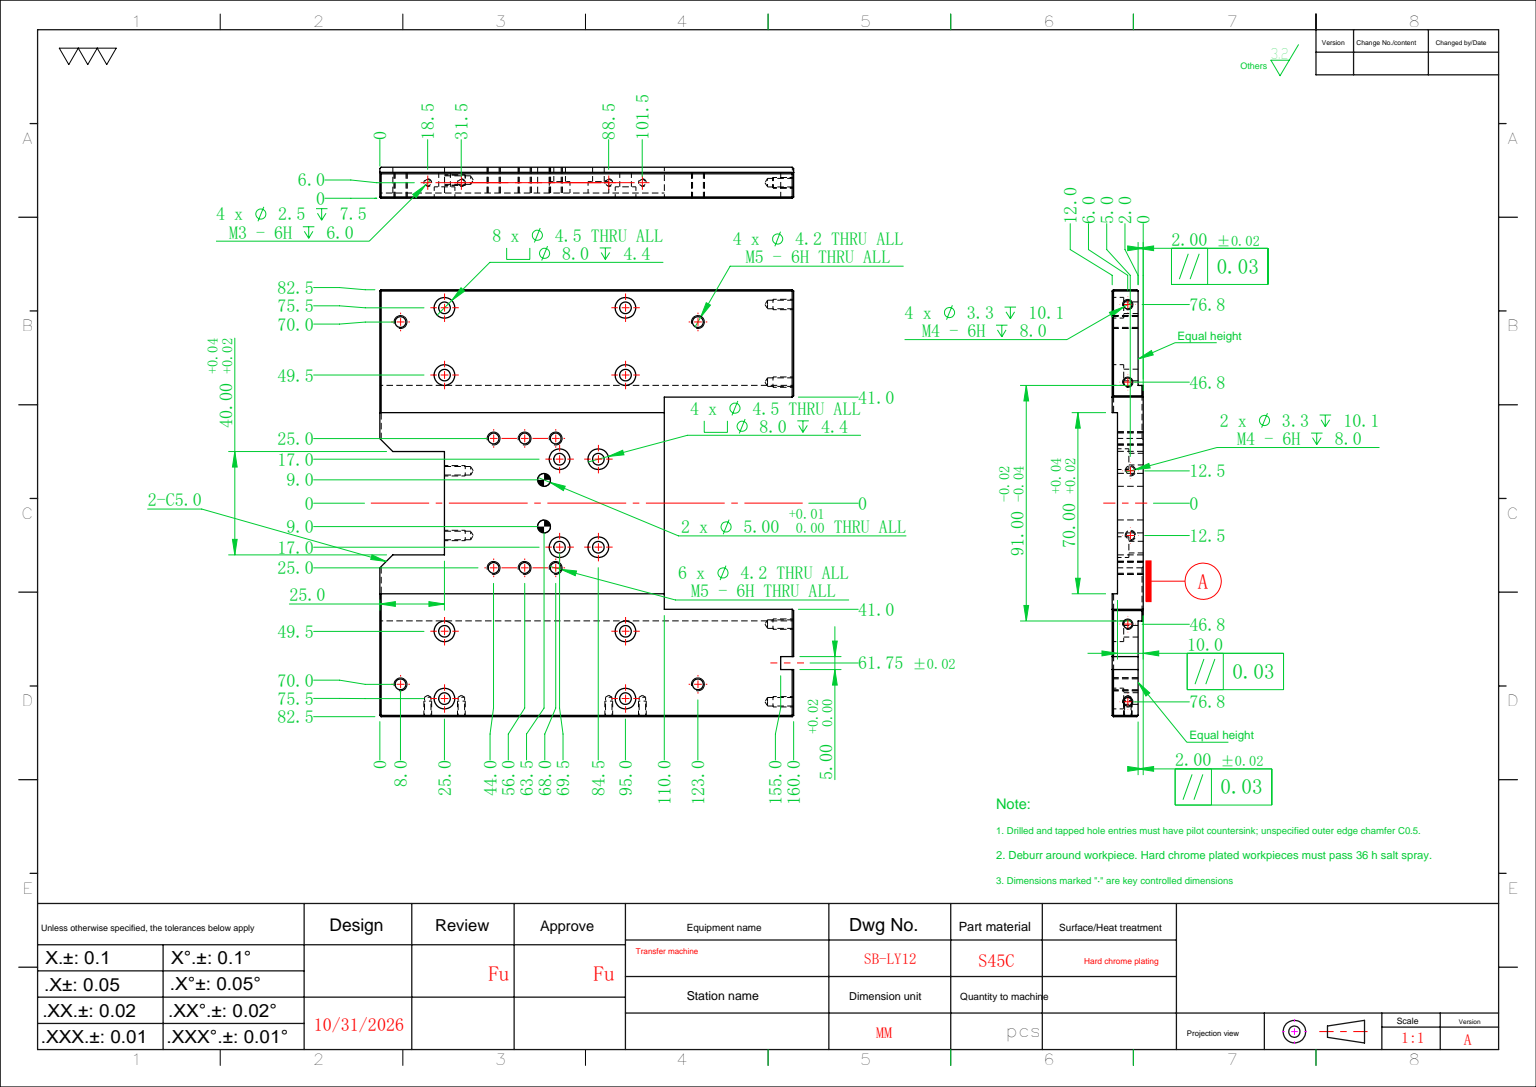
from build123d import *

# Parameters (mm, degrees)
SKETCH_1_W                   = 160
SKETCH_1_H                   = 165
EXTRUDE_1_DEPTH              = 12
SKETCH_2_W                   = 50
SKETCH_2_H                   = 82
CUT_EXTRUDE_1_DEPTH          = 116.543281934
SKETCH_3_W                   = 2
SKETCH_3_H                   = 34
CUT_EXTRUDE_2_DEPTH          = 181.416878368
HOLE_WIZARD_M4_2_D           = 4.5
HOLE_WIZARD_M4_2_CBORE_D     = 8
HOLE_WIZARD_M4_2_CBORE_DEPTH = 4.4
SKETCH_6_W                   = 110
SKETCH_6_H                   = 70
CUT_EXTRUDE_3_DEPTH          = 2
HOLE_WIZARD_M4_1_D           = 4.5
HOLE_WIZARD_M4_1_CBORE_D     = 8
HOLE_WIZARD_M4_1_CBORE_DEPTH = 4.4
MM_2_D                       = 5
HOLE_WIZARD_M5_1_D           = 4.2
HOLE_WIZARD_M4_1_2_D         = 3.3
HOLE_WIZARD_M4_1_2_DEPTH     = 10.1
HOLE_WIZARD_M4_1_2_TIP       = 0.991420021
SKETCH_17_W                  = 10
SKETCH_17_H                  = 5
CUT_EXTRUDE_4_DEPTH          = 5
HOLE_WIZARD_M5_2_D           = 4.2
PATTERN_LINEAR_1_COUNT       = 3
PATTERN_LINEAR_1_PITCH       = 12
SKETCH_20_W                  = 25
SKETCH_20_H                  = 40
CUT_EXTRUDE_5_DEPTH          = 116.543281934
CHAMFER_1_SIZE               = 5
HOLE_WIZARD_M4_2_2_D         = 3.3
HOLE_WIZARD_M4_2_2_DEPTH     = 10.1
HOLE_WIZARD_M4_2_2_TIP       = 0.991420021
HOLE_WIZARD_M3_1_AT_2_COUNT  = 2
HOLE_WIZARD_M3_1_AT_2_PITCH  = 13
PATTERN_LINEAR_2_COUNT       = 2
PATTERN_LINEAR_2_PITCH       = 70
SKETCH_25_W                  = 2
SKETCH_25_H                  = 3
CUT_EXTRUDE_6_DEPTH          = 181.416878368
CHAMFER_2_SIZE               = 0.5


with BuildPart() as part:
    # 草图1 → 凸台-拉伸1 (new body)
    with BuildSketch(Plane.XY):
        Rectangle(SKETCH_1_W, SKETCH_1_H)
    extrude(amount=EXTRUDE_1_DEPTH)

    # 草图2 → 切除-拉伸1 (cut, through all)
    with BuildSketch(Plane(origin=(0, 0, 0), x_dir=(-1, 0, 0), z_dir=(0, 0, -1))):
        with Locations((-55, 0)):
            Rectangle(SKETCH_2_W, SKETCH_2_H)
    extrude(amount=-CUT_EXTRUDE_1_DEPTH, mode=Mode.SUBTRACT)

    # 草图3 → 切除-拉伸2 (cut, through all)
    with BuildSketch(Plane.ZY.offset(80)):
        with Locations((11, 62.5)):
            Rectangle(SKETCH_3_W, SKETCH_3_H)
        with Locations((11, -62.5)):
            Rectangle(SKETCH_3_W, SKETCH_3_H)
    extrude(amount=-CUT_EXTRUDE_2_DEPTH, mode=Mode.SUBTRACT)

    # Hole Wizard M4 _2 (through all)
    with Locations(Plane(origin=(0, 0, 0), x_dir=(-1, 0, 0), z_dir=(0, 0, -1))):
        with Locations((-15, 49.5), (-15, 75.5), (-15, -75.5), (-15, -49.5), (55, -75.5), (55, -49.5), (55, 49.5), (55, 75.5)):
            CounterBoreHole(HOLE_WIZARD_M4_2_D / 2, HOLE_WIZARD_M4_2_CBORE_D / 2, HOLE_WIZARD_M4_2_CBORE_DEPTH)

    # 草图6 → 切除-拉伸3 (cut)
    with BuildSketch(Plane(origin=(0, 0, 0), x_dir=(-1, 0, 0), z_dir=(0, 0, -1))):
        with Locations((25, 0)):
            Rectangle(SKETCH_6_W, SKETCH_6_H)
    extrude(amount=-CUT_EXTRUDE_3_DEPTH, mode=Mode.SUBTRACT)

    # Hole Wizard M4 _1 (through all)
    with Locations(Plane(origin=(0, 0, 2), x_dir=(-1, 0, 0), z_dir=(0, 0, -1))):
        with Locations((-4.5, -17), (-4.5, 17), (10.5, -17), (10.5, 17)):
            CounterBoreHole(HOLE_WIZARD_M4_1_D / 2, HOLE_WIZARD_M4_1_CBORE_D / 2, HOLE_WIZARD_M4_1_CBORE_DEPTH)

    # 大小mm 暗销孔2 (through all)
    with Locations(Plane(origin=(0, 0, 2), x_dir=(-1, 0, 0), z_dir=(0, 0, -1))):
        with Locations((16.5, -9), (16.5, 9)):
            Hole(MM_2_D / 2)

    # M5 螺纹孔1 (through all)
    with Locations(Plane(origin=(0, 0, 0), x_dir=(-1, 0, 0), z_dir=(0, 0, -1))):
        with Locations((72, 70), (-43, 70), (-43, -70), (72, -70)):
            Hole(HOLE_WIZARD_M5_1_D / 2)

    # Hole Wizard M4 _1 2
    with Locations(Plane(origin=(80, 0, 0), x_dir=(0, 0, -1), z_dir=(1, 0, 0))):
        with Locations((-6, 76.75), (-6, 46.75), (-6, -46.75), (-6, -76.75)):
            Hole(HOLE_WIZARD_M4_1_2_D / 2, depth=HOLE_WIZARD_M4_1_2_DEPTH)
            with Locations((0, 0, -(HOLE_WIZARD_M4_1_2_DEPTH + HOLE_WIZARD_M4_1_2_TIP / 2))):  # 118° drill point
                Cone(0, HOLE_WIZARD_M4_1_2_D / 2, HOLE_WIZARD_M4_1_2_TIP, mode=Mode.SUBTRACT)

    # 草图17 → 切除-拉伸4 (cut)
    with BuildSketch(Plane(origin=(80, 0, 0), x_dir=(0, 0, -1), z_dir=(1, 0, 0))):
        with Locations((-5, 61.75)):
            Rectangle(SKETCH_17_W, SKETCH_17_H)
    extrude(amount=-CUT_EXTRUDE_4_DEPTH, mode=Mode.SUBTRACT)

    # M5 螺纹孔2 (through all)
    with Locations(Plane(origin=(0, 0, 2), x_dir=(-1, 0, 0), z_dir=(0, 0, -1))):
        with Locations((12, 25), (12, -25)):
            hole_wizard_m5_2 = Hole(HOLE_WIZARD_M5_2_D / 2)

    # 阵列(线性)1: M5 螺纹孔2 ×3
    with Locations(*[(-i * PATTERN_LINEAR_1_PITCH, 0, 0) for i in range(1, PATTERN_LINEAR_1_COUNT)]):
        add(hole_wizard_m5_2, mode=Mode.SUBTRACT)

    # 草图20 → 切除-拉伸5 (cut, through all)
    with BuildSketch(Plane(origin=(0, 0, 0), x_dir=(-1, 0, 0), z_dir=(0, 0, -1))):
        with Locations((67.5, 0)):
            Rectangle(SKETCH_20_W, SKETCH_20_H)
    extrude(amount=-CUT_EXTRUDE_5_DEPTH, mode=Mode.SUBTRACT)

    # 倒角1
    chamfer_1_edges = [part.edges().sort_by_distance(p)[0] for p in [
        (-80, 20, 7),
        (-80, -20, 7),
    ]]
    chamfer(chamfer_1_edges, length=CHAMFER_1_SIZE)

    # Hole Wizard M4 _2 2
    with Locations(Plane.ZY.offset(55)):
        with Locations((7, 12.5), (7, -12.5)):
            Hole(HOLE_WIZARD_M4_2_2_D / 2, depth=HOLE_WIZARD_M4_2_2_DEPTH)
            with Locations((0, 0, -(HOLE_WIZARD_M4_2_2_DEPTH + HOLE_WIZARD_M4_2_2_TIP / 2))):  # 118° drill point
                Cone(0, HOLE_WIZARD_M4_2_2_D / 2, HOLE_WIZARD_M4_2_2_TIP, mode=Mode.SUBTRACT)

    # 草图24 → M3 螺纹孔1 (revolve, cut)
    with BuildSketch(Plane(origin=(-61.5, 82.5, 6), x_dir=(0, 0, 1), z_dir=(1, 0, 0))):
        Polygon((0, 0), (0, 8.251075774), (1.25, 7.5), (1.25, 0), align=None)
    hole_wizard_m3_1 = revolve(axis=Axis((-61.5, 88.85, 6), (0, -1, 0)), mode=Mode.SUBTRACT)

    # M3 螺纹孔1 at 2: M3 螺纹孔1 ×2
    with Locations(*[(i * HOLE_WIZARD_M3_1_AT_2_PITCH, 0, 0) for i in range(1, HOLE_WIZARD_M3_1_AT_2_COUNT)]):
        add(hole_wizard_m3_1, mode=Mode.SUBTRACT)

    # 阵列(线性)2: M3 螺纹孔1 ×2
    with Locations(*[(i * PATTERN_LINEAR_2_PITCH, 0, 0) for i in range(1, PATTERN_LINEAR_2_COUNT)]):
        add(hole_wizard_m3_1, mode=Mode.SUBTRACT)

    # 阵列(线性)2 copy 1 sketch → 阵列(线性)2 copy 1 (revolve, cut)
    with BuildSketch(Plane(origin=(21.5, 82.5, 6), x_dir=(0, 0, 1), z_dir=(1, 0, 0))):
        Polygon((0, 0), (0, 8.251075774), (1.25, 7.5), (1.25, 0), align=None)
    revolve(axis=Axis((21.5, 88.85, 6), (0, -1, 0)), mode=Mode.SUBTRACT)

    # 草图25 → 切除-拉伸6 (cut, through all)
    with BuildSketch(Plane(origin=(80, 0, 0), x_dir=(0, 0, -1), z_dir=(1, 0, 0))):
        with Locations((-11, 81)):
            Rectangle(SKETCH_25_W, SKETCH_25_H)
        with Locations((-11, -81)):
            Rectangle(SKETCH_25_W, SKETCH_25_H)
    extrude(amount=-CUT_EXTRUDE_6_DEPTH, mode=Mode.SUBTRACT)

    # 倒角2
    chamfer_2_edges = [part.edges().sort_by_distance(p)[0] for p in [
        (-80, -58.75, 0),
        (80, 50.125, 0),
        (80, 43.25, 12),
        (80, -41, 6),
        (80, 41, 6),
        (80, 73.375, 0),
        (-80, -35.25, 12),
        (-80, 35.25, 12),
        (80, -43.25, 12),
        (80, -82.5, 5),
        (-80, -82.5, 5),
        (-80, 82.5, 5),
        (80, 82.5, 5),
        (0, 82.5, 10),
        (0, -82.5, 10),
        (0, -82.5, 0),
        (-80, 58.75, 0),
        (0, 82.5, 0),
        (80, -61.75, 0),
    ]]
    chamfer(chamfer_2_edges, length=CHAMFER_2_SIZE)


solid = part.part
